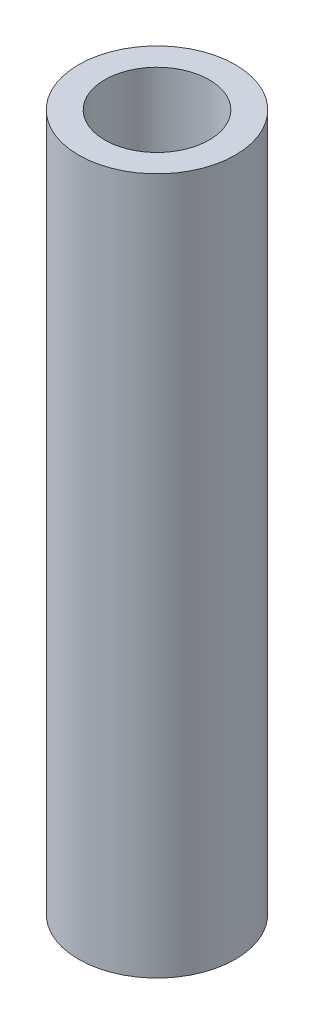
SolidWorks part; units mm, degrees
ref_plane "Front Plane" through (0, 0, 0) normal (0, 0, 1) x (1, 0, 0)
ref_plane "Top Plane" through (0, 0, 0) normal (0, 1, 0) x (1, 0, 0)
ref_plane "Right Plane" through (0, 0, 0) normal (1, 0, 0) x (0, 0, -1)
sketch "Sketch1" plane through (0, 0, 0) normal (0, 1, 0) x (1, 0, 0)
  circle A0 centre (0, 0) radius 2.25
  circle A1 centre (0, 0) radius 1.5
  dimension "D1" = 4.5
  dimension "D2" = 3
extrude "Boss-Extrude1" add sketch "Sketch1" along normal blind 20
